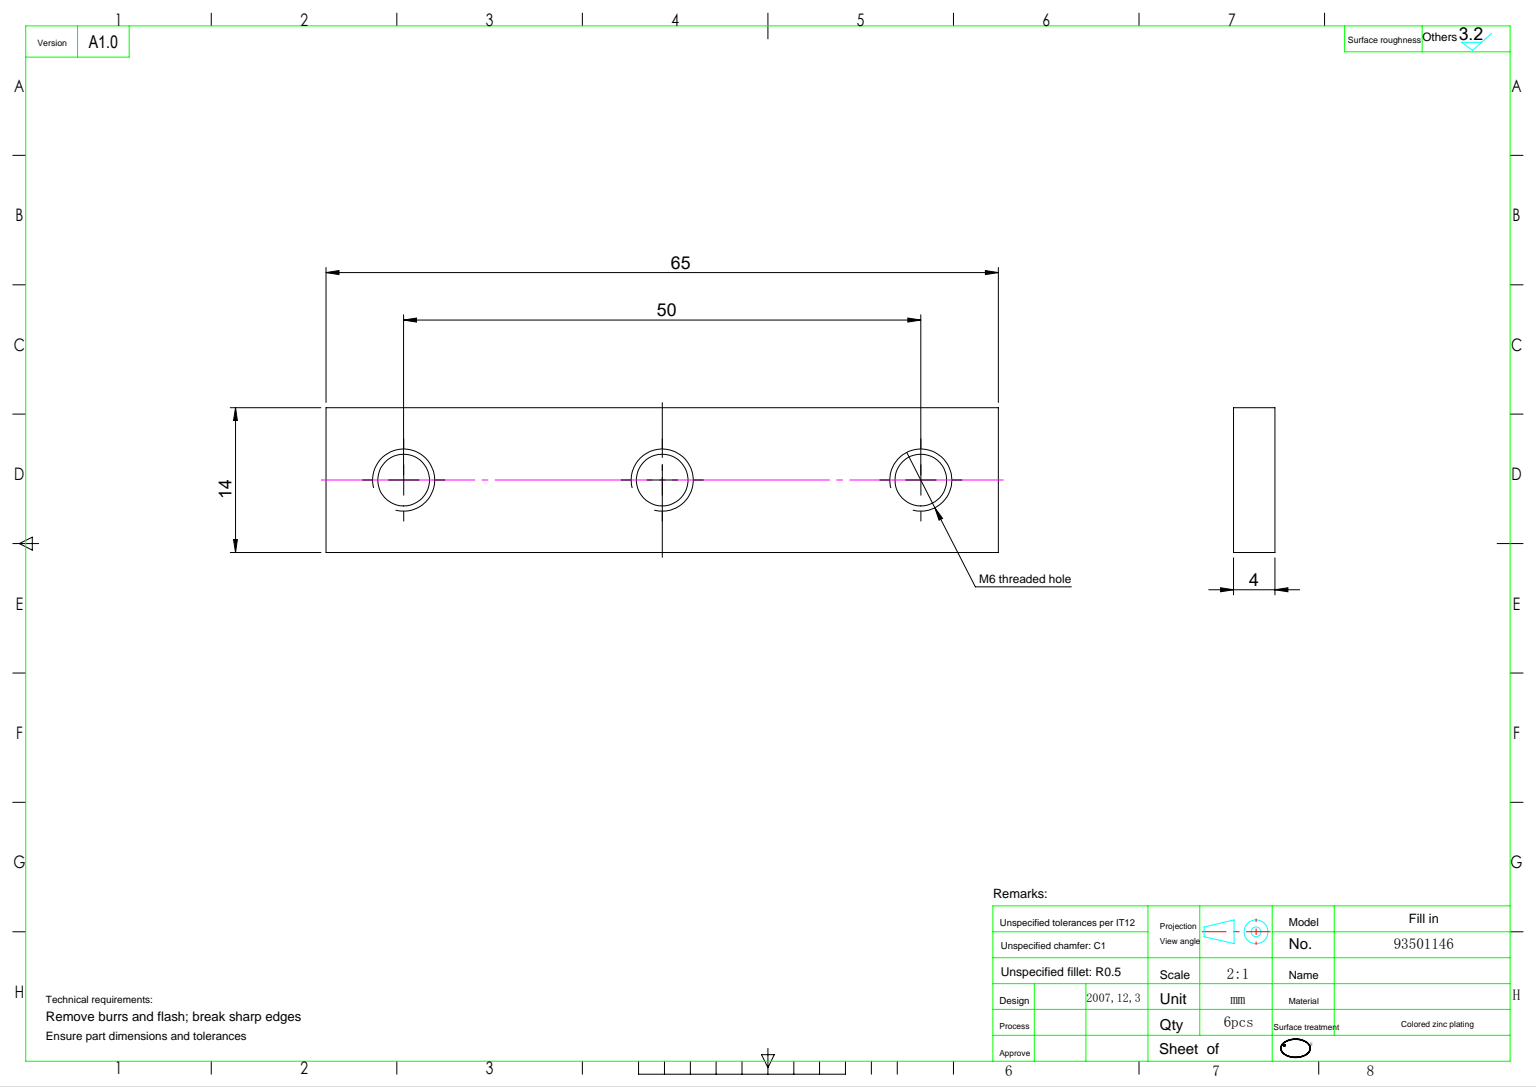
from build123d import *

# Parameters (mm, degrees)
SKETCH_2_W         = 65
SKETCH_2_H         = 14
EXTRUDE_1_DEPTH    = 2
HOLE_WIZARD_M6_1_D = 5


with BuildPart() as part:
    # 草图2 → 凸台-拉伸1 (new, symmetric)
    with BuildSketch(Plane(origin=(0, 0, 0), x_dir=(1, 0, 0), z_dir=(0, 1, 0))):
        Rectangle(SKETCH_2_W, SKETCH_2_H)
    extrude(amount=EXTRUDE_1_DEPTH, both=True)

    # M6 螺纹孔1 (through all)
    with Locations(Plane(origin=(0, 2, 0), x_dir=(1, 0, 0), z_dir=(0, 1, 0))):
        with Locations((-25, 0), (0, 0), (25, 0)):
            Hole(HOLE_WIZARD_M6_1_D / 2)


solid = part.part
